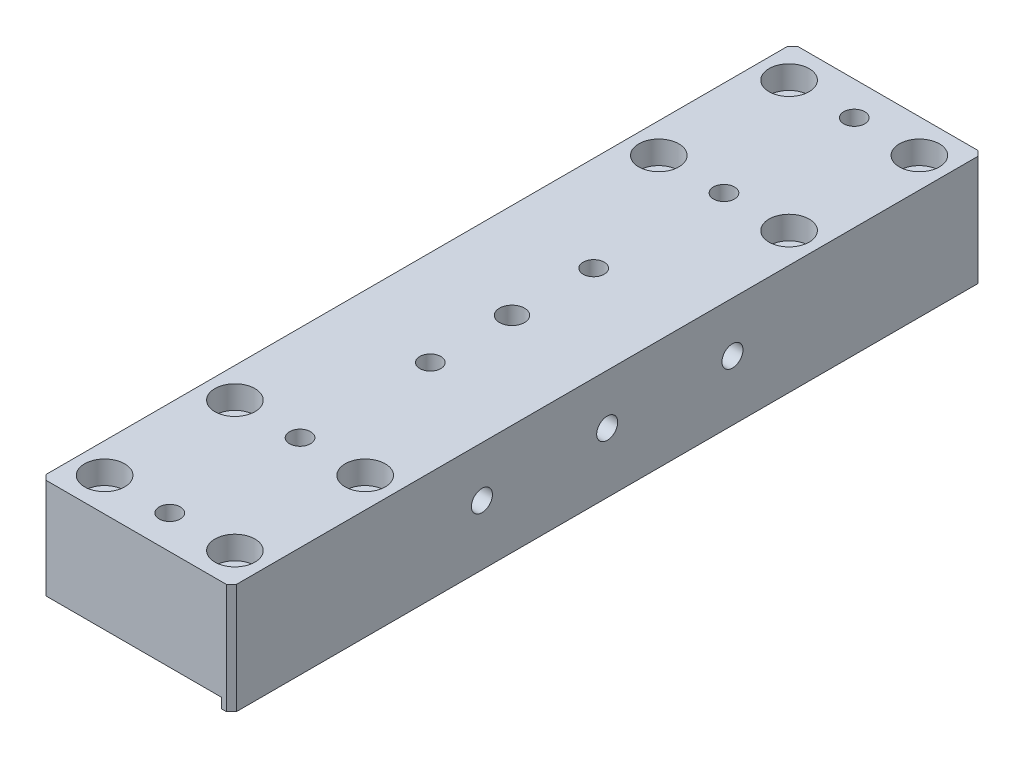
SolidWorks part; units mm, degrees
material "AL6061"
ref_plane "Front" through (0, 0, 0) normal (0, 0, 1) x (1, 0, 0)
ref_plane "Top" through (0, 0, 0) normal (0, 1, 0) x (1, 0, 0)
ref_plane "Right" through (0, 0, 0) normal (1, 0, 0) x (0, 0, -1)
sketch "Sketch1" plane through (0, 0, 0) normal (0, 0, 1) x (1, 0, 0)
  line L0 (0, 0) -> (0, 22)
  line L1 (0, 22) -> (-38, 22)
  line L2 (-38, 22) -> (-38, 2)
  line L3 (-38, 2) -> (-2, 2)
  line L4 (-2, 2) -> (-2, 0)
  line L5 (-2, 0) -> (0, 0)
  dimension "D1" = 20
  dimension "D2" = 38
  dimension "D3" = 2
  dimension "D4" = 2
extrude "Boss-Extrude1" add sketch "Sketch1" along normal mid plane 150
hole_wizard "Hole size (socket head cap screw type)1" positions "Sketch2" profile "Sketch3" counterbore size "M4" standard "GB" end condition through all
sketch "Sketch2" plane through (0, 22, 0) normal (0, 1, 0) x (1, 0, 0)
  line L0 (0, 0) -> (-52.7578, 0) construction
  line L4 (-32, 68.3) -> (-6, 68.3)
  line L5 (-32, 68.3) -> (-32, 42.3)
  line L6 (-32, 42.3) -> (-6, 42.3)
  line L7 (-6, 68.3) -> (-6, 42.3)
  line L8 (-6, -68.3) -> (-6, -42.3)
  line L9 (-32, -42.3) -> (-6, -42.3)
  line L10 (-32, -68.3) -> (-32, -42.3)
  line L11 (-32, -68.3) -> (-6, -68.3)
  line L12 (-2, -75) -> (-2, 75) construction
  point P8 (-32, 68.3)
  point P9 (-6, 42.3)
  point P170 (-32, 42.3)
  point P171 (-6, 68.3)
  point P172 (-6, -68.3)
  point P173 (-6, -42.3)
  point P174 (-32, -42.3)
  point P175 (-32, -68.3)
  dimension "D1" = 110.6
  dimension "D2" = 26
  dimension "D3" = 4
sketch "Sketch3" plane through (-32, 22, 68.3) normal (1, 0, 0) x (0, 0, 1)
  line L0 (0, 0) -> (0, 22)
  line L1 (0, 22) -> (2.25, 22)
  line L3 (2.25, 22) -> (2.25, 4.6)
  line L4 (2.25, 4.6) -> (4, 4.6)
  line L5 (4, 4.6) -> (4, 0)
  line L7 (4, 0) -> (0, 0)
  line L11 (0, -6.35) -> (0, 107.95) construction
  dimension "通孔孔直径" = 4.5
  dimension "通孔孔深度" = 22
  dimension "柱形沉头孔直径" = 8
  dimension "柱形沉头孔深度" = 4.6
hole_wizard "M5 Tapped Hole1" positions "Sketch4" profile "Sketch5" tap size "M5" standard "GB"
sketch "Sketch4" plane through (0, 0, 0) normal (1, 0, 0) x (0, 0, -1)
  line L0 (0, 0) -> (0, 30.7571) construction
  line L3 (-78.5654, 12) -> (85.5113, 12) construction
  line L4 (-75, 22) -> (75, 22) construction
  point P13 (-25, 12)
  point P16 (25, 12)
  point P17 (0, 12)
  dimension "D1" = 50
  dimension "D2" = 10
sketch "Sketch5" plane through (0, 12, 0) normal (0, 1, 0) x (0, 0, -1)
  line L0 (0, 0) -> (0, 13.6618)
  line L1 (0, 13.6618) -> (2.1, 12.4)
  line L2 (2.1, 12.4) -> (2.1, 0)
  line L5 (2.1, 0) -> (0, 0)
  line L10 (0, 13.6618) -> (-2.1, 12.4) construction
  line L11 (0, -6.35) -> (0, 107.95) construction
  dimension "螺纹孔钻头直径" = 4.2
  dimension "螺纹孔钻头深度" = 12.4
  dimension "导头角度" = 118
cosmetic thread "Cosmetic Thread1" parameters "D1"=10, "D2"=5
cosmetic thread "Cosmetic Thread2" parameters "D1"=10, "D2"=5
cosmetic thread "Cosmetic Thread3" parameters "D1"=10, "D2"=5
hole_wizard "M5 Tapped Hole2" positions "Sketch8" profile "Sketch9" tap size "M5" standard "GB"
sketch "Sketch8" plane through (0, 22, 0) normal (0, 1, 0) x (1, 0, 0)
  line L0 (0, 0) -> (-54.3558, 0) construction
  line L3 (-19, 75) -> (-19, -82.8964) construction
  line L4 (0, 75) -> (-38, 75) construction
  line L5 (-32, 68.3) -> (-6, 68.3) construction
  line L8 (-32, 42.3) -> (-6, 42.3) construction
  point P15 (-19, 68.3)
  point P17 (-19, 42.3)
  point P22 (-19, -42.3)
  point P23 (-19, -68.3)
  point P46 (-19, 16.3)
  point P49 (-19, -16.3)
  dimension "D1" = 26
sketch "Sketch9" plane through (-19, 22, 16.3) normal (1, 0, 0) x (0, 0, 1)
  line L0 (0, 0) -> (0, 13.6618)
  line L1 (0, 13.6618) -> (2.1, 12.4)
  line L2 (2.1, 12.4) -> (2.1, 0)
  line L5 (2.1, 0) -> (0, 0)
  line L10 (0, 13.6618) -> (-2.1, 12.4) construction
  line L11 (0, -6.35) -> (0, 107.95) construction
  dimension "螺纹孔钻头直径" = 4.2
  dimension "螺纹孔钻头深度" = 12.4
  dimension "导头角度" = 118
cosmetic thread "Cosmetic Thread4" parameters "D1"=10, "D2"=5
cosmetic thread "Cosmetic Thread5" parameters "D1"=10, "D2"=5
cosmetic thread "Cosmetic Thread6" parameters "D1"=10, "D2"=5
cosmetic thread "Cosmetic Thread7" parameters "D1"=10, "D2"=5
cosmetic thread "Cosmetic Thread8" parameters "D1"=10, "D2"=5
cosmetic thread "Cosmetic Thread9" parameters "D1"=10, "D2"=5
chamfer "Chamfer1" distance 1 angle 45 4 edges at (0, 11, 75) (-38, 12, 75) (-38, 12, -75) (0, 11, -75)
hole_wizard "Dowel Hole1" positions "Sketch10" profile "Sketch11" hole size "Ø5.0" standard "GB"
sketch "Sketch10" plane through (0, 22, 0) normal (0, 1, 0) x (1, 0, 0)
  line L0 (-19, 16.3) -> (-19, -16.3) construction
  point P9 (-19, 0)
sketch "Sketch11" plane through (-19, 22, 0) normal (1, 0, 0) x (0, 0, 1)
  line L0 (0, 0) -> (0, 9.0022)
  line L1 (0, 9.0022) -> (2.5, 7.5)
  line L2 (2.5, 7.5) -> (2.5, 0)
  line L5 (2.5, 0) -> (0, 0)
  line L10 (0, 9.0022) -> (-2.5, 7.5) construction
  line L11 (0, -6.35) -> (0, 107.95) construction
  dimension "孔直径" = 5
  dimension "孔深度" = 7.5
  dimension "导头角度" = 118
